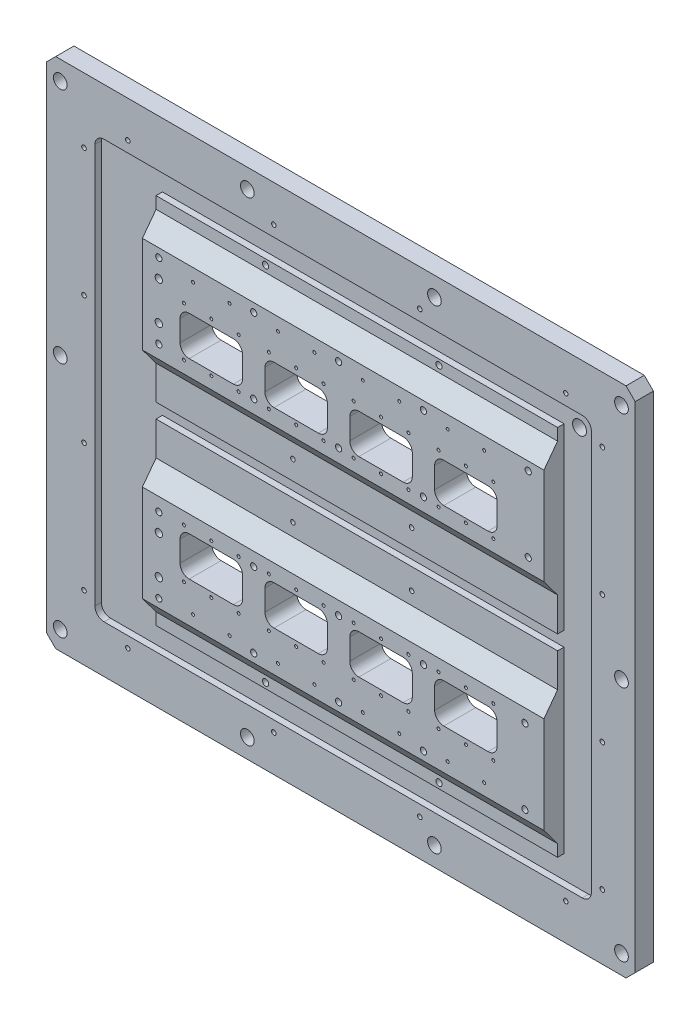
from build123d import *

# Parameters (mm, degrees)
SKETCH1_W             = 645
SKETCH1_H             = 562
BOSS_EXTRUDE1_DEPTH   = 20
SKETCH2_W             = 544
SKETCH2_H             = 458
CUT_EXTRUDE1_DEPTH    = 7
CHAMFER1_SIZE         = 10
BOSS_EXTRUDE2_DEPTH   = 440
CUT_EXTRUDE2_DEPTH    = 440
HOLE1_D               = 8.4
HOLE1_CBORE_D         = 15
HOLE1_CBORE_DEPTH     = 11
FILLET1_R             = 10
M6_TAPPED_HOLE1_D     = 5
M6_TAPPED_HOLE1_DEPTH = 10
M6_TAPPED_HOLE1_TIP   = 1.502151548
G3_8_TAPPED_HOLE1_D   = 15.25
M8_TAPPED_HOLE1_D     = 6.8
M8_TAPPED_HOLE1_DEPTH = 16
M8_TAPPED_HOLE1_TIP   = 2.042926105
HOLE2_D               = 8
HOLE2_DEPTH           = 8.5
M8_TAPPED_HOLE2_D     = 6.8
M8_TAPPED_HOLE2_DEPTH = 16
M8_TAPPED_HOLE2_TIP   = 2.042926105
M4_TAPPED_HOLE1_D     = 3.3
M4_TAPPED_HOLE1_DEPTH = 8
M4_TAPPED_HOLE1_TIP   = 0.991420021
M4_TAPPED_HOLE2_D     = 3.3
M4_TAPPED_HOLE2_DEPTH = 8
M4_TAPPED_HOLE2_TIP   = 0.991420021
M6_TAPPED_HOLE2_D     = 5
M6_TAPPED_HOLE2_DEPTH = 12
M6_TAPPED_HOLE2_TIP   = 1.502151548
M8_TAPPED_HOLE3_D     = 6.8
M8_TAPPED_HOLE3_DEPTH = 16
M8_TAPPED_HOLE3_TIP   = 2.042926105


with BuildPart() as part:
    # Sketch1 → Boss-Extrude1 (new body)
    with BuildSketch(Plane.XY):
        Rectangle(SKETCH1_W, SKETCH1_H)
    extrude(amount=BOSS_EXTRUDE1_DEPTH)

    # Sketch2 → Cut-Extrude1 (cut)
    with BuildSketch(Plane.XY.offset(20)):
        with Locations((2.5, 0)):
            Rectangle(SKETCH2_W, SKETCH2_H)
    extrude(amount=-CUT_EXTRUDE1_DEPTH, mode=Mode.SUBTRACT)

    # Chamfer1
    chamfer1_edges = [part.edges().sort_by_distance(p)[0] for p in [
        (322.5, -281, 10),
        (-322.5, -281, 10),
        (-322.5, 281, 10),
        (322.5, 281, 10),
    ]]
    chamfer(chamfer1_edges, length=CHAMFER1_SIZE)

    # Sketch3 → Boss-Extrude2 (add)
    with BuildSketch(Plane(origin=(-202.5, 0, 0), x_dir=(0, 0, -1), z_dir=(1, 0, 0))):
        Polygon((-13, 204), (-20, 204), (-20, 191), (-35, 171), (-35, 65), (-20, 45), (-20, 8), (-13, 8), align=None)
        Polygon((-20, -8), (-20, -45), (-35, -65), (-35, -171), (-20, -191), (-20, -204), (-13, -204), (-13, -8), align=None)
    extrude(amount=BOSS_EXTRUDE2_DEPTH)

    # Sketch4 → Cut-Extrude2 (cut)
    with BuildSketch(Plane.XY.offset(35)):
        with BuildLine():
            Line((-151.25, -83.74), (-102.75, -83.74))
            ThreePointArc((-102.75, -83.74), (-95.678932188, -86.668932188), (-92.75, -93.74))
            Line((-92.75, -93.74), (-92.75, -116.74))
            ThreePointArc((-92.75, -116.74), (-95.678932188, -123.811067812), (-102.75, -126.74))
            Line((-102.75, -126.74), (-151.25, -126.74))
            ThreePointArc((-151.25, -126.74), (-158.321067812, -123.811067812), (-161.25, -116.74))
            Line((-161.25, -116.74), (-161.25, -93.74))
            ThreePointArc((-161.25, -93.74), (-158.321067812, -86.668932188), (-151.25, -83.74))
        make_face()
        with BuildLine():
            Line((-68.25, -93.74), (-68.25, -116.74))
            ThreePointArc((-68.25, -116.74), (-65.321067812, -123.811067812), (-58.25, -126.74))
            Line((-58.25, -126.74), (-9.75, -126.74))
            ThreePointArc((-9.75, -126.74), (-2.678932188, -123.811067812), (0.25, -116.74))
            Line((0.25, -116.74), (0.25, -93.74))
            ThreePointArc((0.25, -93.74), (-2.678932188, -86.668932188), (-9.75, -83.74))
            Line((-9.75, -83.74), (-58.25, -83.74))
            ThreePointArc((-58.25, -83.74), (-65.321067812, -86.668932188), (-68.25, -93.74))
        make_face()
        with BuildLine():
            Line((24.75, -93.74), (24.75, -116.74))
            ThreePointArc((24.75, -116.74), (27.678932188, -123.811067812), (34.75, -126.74))
            Line((34.75, -126.74), (83.25, -126.74))
            ThreePointArc((83.25, -126.74), (90.321067812, -123.811067812), (93.25, -116.74))
            Line((93.25, -116.74), (93.25, -93.74))
            ThreePointArc((93.25, -93.74), (90.321067812, -86.668932188), (83.25, -83.74))
            Line((83.25, -83.74), (34.75, -83.74))
            ThreePointArc((34.75, -83.74), (27.678932188, -86.668932188), (24.75, -93.74))
        make_face()
        with BuildLine():
            Line((117.75, -93.74), (117.75, -116.74))
            ThreePointArc((117.75, -116.74), (120.678932188, -123.811067812), (127.75, -126.74))
            Line((127.75, -126.74), (176.25, -126.74))
            ThreePointArc((176.25, -126.74), (183.321067812, -123.811067812), (186.25, -116.74))
            Line((186.25, -116.74), (186.25, -93.74))
            ThreePointArc((186.25, -93.74), (183.321067812, -86.668932188), (176.25, -83.74))
            Line((176.25, -83.74), (127.75, -83.74))
            ThreePointArc((127.75, -83.74), (120.678932188, -86.668932188), (117.75, -93.74))
        make_face()
        with BuildLine():
            Line((-68.25, 115.5), (-68.25, 92.5))
            ThreePointArc((-68.25, 92.5), (-65.321067812, 85.428932188), (-58.25, 82.5))
            Line((-58.25, 82.5), (-9.75, 82.5))
            ThreePointArc((-9.75, 82.5), (-2.678932188, 85.428932188), (0.25, 92.5))
            Line((0.25, 92.5), (0.25, 115.5))
            ThreePointArc((0.25, 115.5), (-2.678932188, 122.571067812), (-9.75, 125.5))
            Line((-9.75, 125.5), (-58.25, 125.5))
            ThreePointArc((-58.25, 125.5), (-65.321067812, 122.571067812), (-68.25, 115.5))
        make_face()
        with BuildLine():
            Line((24.75, 115.5), (24.75, 92.5))
            ThreePointArc((24.75, 92.5), (27.678932188, 85.428932188), (34.75, 82.5))
            Line((34.75, 82.5), (83.25, 82.5))
            ThreePointArc((83.25, 82.5), (90.321067812, 85.428932188), (93.25, 92.5))
            Line((93.25, 92.5), (93.25, 115.5))
            ThreePointArc((93.25, 115.5), (90.321067812, 122.571067812), (83.25, 125.5))
            Line((83.25, 125.5), (34.75, 125.5))
            ThreePointArc((34.75, 125.5), (27.678932188, 122.571067812), (24.75, 115.5))
        make_face()
        with BuildLine():
            Line((117.75, 115.5), (117.75, 92.5))
            ThreePointArc((117.75, 92.5), (120.678932188, 85.428932188), (127.75, 82.5))
            Line((127.75, 82.5), (176.25, 82.5))
            ThreePointArc((176.25, 82.5), (183.321067812, 85.428932188), (186.25, 92.5))
            Line((186.25, 92.5), (186.25, 115.5))
            ThreePointArc((186.25, 115.5), (183.321067812, 122.571067812), (176.25, 125.5))
            Line((176.25, 125.5), (127.75, 125.5))
            ThreePointArc((127.75, 125.5), (120.678932188, 122.571067812), (117.75, 115.5))
        make_face()
        with BuildLine():
            Line((-161.25, 115.5), (-161.25, 92.5))
            ThreePointArc((-161.25, 92.5), (-158.321067812, 85.428932188), (-151.25, 82.5))
            Line((-151.25, 82.5), (-102.75, 82.5))
            ThreePointArc((-102.75, 82.5), (-95.678932188, 85.428932188), (-92.75, 92.5))
            Line((-92.75, 92.5), (-92.75, 115.5))
            ThreePointArc((-92.75, 115.5), (-95.678932188, 122.571067812), (-102.75, 125.5))
            Line((-102.75, 125.5), (-151.25, 125.5))
            ThreePointArc((-151.25, 125.5), (-158.321067812, 122.571067812), (-161.25, 115.5))
        make_face()
    extrude(amount=-CUT_EXTRUDE2_DEPTH, mode=Mode.SUBTRACT)

    # Hole1 (through all)
    with Locations(Plane.XY.offset(20)):
        with Locations((-307.5, 260), (-102.5, 260), (102.5, 260), (307.5, 260), (307.5, 0), (307.5, -260), (102.5, -260), (-102.5, -260), (-307.5, -260), (-307.5, 0)):
            CounterBoreHole(HOLE1_D / 2, HOLE1_CBORE_D / 2, HOLE1_CBORE_DEPTH)

    # Fillet1
    fillet1_edges = [part.edges().sort_by_distance(p)[0] for p in [
        (-269.5, -229, 16.5),
        (-269.5, 229, 16.5),
        (274.5, 229, 16.5),
        (274.5, -229, 16.5),
    ]]
    fillet(fillet1_edges, radius=FILLET1_R)

    # M6 Tapped Hole1
    with Locations(Plane.XY.offset(20)):
        with Locations((-281.5, -210), (-233.5, -241), (-73.5, -241), (86.5, -241), (246.5, -241), (286.5, 70), (286.5, 210), (246.5, 241), (86.5, 241), (-73.5, 241), (-233.5, 241), (-281.5, 210), (-281.5, 70), (286.5, -210), (286.5, -70), (-281.5, -70)):
            Hole(M6_TAPPED_HOLE1_D / 2, depth=M6_TAPPED_HOLE1_DEPTH)
            with Locations((0, 0, -(M6_TAPPED_HOLE1_DEPTH + M6_TAPPED_HOLE1_TIP / 2))):  # 118° drill point
                Cone(0, M6_TAPPED_HOLE1_D / 2, M6_TAPPED_HOLE1_TIP, mode=Mode.SUBTRACT)

    # G3/8 Tapped Hole1 (through all)
    with Locations(Plane.XY.offset(13)):
        with Locations((254.5, 209)):
            Hole(G3_8_TAPPED_HOLE1_D / 2)

    # M8 Tapped Hole1
    with Locations(Plane(origin=(0, 0, 0), x_dir=(-1, 0, 0), z_dir=(0, 0, -1))):
        with Locations((-212.5, 170), (-112.5, 170), (-12.5, 170), (87.5, 170), (187.5, 170), (187.5, 28), (87.5, 28), (-12.5, 28), (-112.5, 28), (-212.5, 28), (-212.5, -24), (-212.5, -166), (-112.5, -166), (-112.5, -24), (-12.5, -24), (87.5, -24), (187.5, -24), (187.5, -166), (87.5, -166), (-12.5, -166)):
            Hole(M8_TAPPED_HOLE1_D / 2, depth=M8_TAPPED_HOLE1_DEPTH)
            with Locations((0, 0, -(M8_TAPPED_HOLE1_DEPTH + M8_TAPPED_HOLE1_TIP / 2))):  # 118° drill point
                Cone(0, M8_TAPPED_HOLE1_D / 2, M8_TAPPED_HOLE1_TIP, mode=Mode.SUBTRACT)

    # Hole2
    with Locations(Plane.XY.offset(35)):
        with Locations((-184.5, 141.6), (-184.5, 99.6), (-184.5, -99.6), (-184.5, -141.6)):
            Hole(HOLE2_D / 2, depth=HOLE2_DEPTH)

    # M8 Tapped Hole2
    with Locations(Plane.XY.offset(35)):
        with Locations((-184.5, 161.6), (-80.5, 161.6), (12.5, 161.6), (105.5, 161.6), (220.3, 161.6), (220.3, 79.6), (105.5, 79.6), (12.5, 79.6), (-80.5, 79.6), (-184.5, 79.6), (-184.5, -79.6), (-184.5, -161.6), (-80.5, -161.6), (-80.5, -79.6), (12.5, -79.6), (12.5, -161.6), (105.5, -161.6), (105.5, -79.6), (216.7, -79.6), (216.7, -161.6)):
            Hole(M8_TAPPED_HOLE2_D / 2, depth=M8_TAPPED_HOLE2_DEPTH)
            with Locations((0, 0, -(M8_TAPPED_HOLE2_DEPTH + M8_TAPPED_HOLE2_TIP / 2))):  # 118° drill point
                Cone(0, M8_TAPPED_HOLE2_D / 2, M8_TAPPED_HOLE2_TIP, mode=Mode.SUBTRACT)

    # M4 Tapped Hole1
    with Locations(Plane.XY.offset(35)):
        with Locations((-147, 157), (-107, 157), (-54, 157), (-14, 157), (39, 157), (79, 157), (132, 157), (172, 157), (-147, -158.24), (-107, -158.24), (-54, -158.24), (-14, -158.24), (39, -158.24), (79, -158.24), (132, -158.24), (172, -158.24)):
            Hole(M4_TAPPED_HOLE1_D / 2, depth=M4_TAPPED_HOLE1_DEPTH)
            with Locations((0, 0, -(M4_TAPPED_HOLE1_DEPTH + M4_TAPPED_HOLE1_TIP / 2))):  # 118° drill point
                Cone(0, M4_TAPPED_HOLE1_D / 2, M4_TAPPED_HOLE1_TIP, mode=Mode.SUBTRACT)

    # M4 Tapped Hole2
    with Locations(Plane.XY.offset(35)):
        with Locations((-157, -78.24), (-127, -78.24), (-97, -78.24), (-157, -132.24), (-127, -132.24), (-97, -132.24), (-64, -78.24), (-34, -78.24), (-4, -78.24), (-34, -132.24), (-64, -132.24), (-4, -132.24), (29, -78.24), (59, -78.24), (89, -78.24), (122, -78.24), (122, -132.24), (89, -132.24), (59, -132.24), (29, -132.24), (152, -78.24), (182, -78.24), (182, -132.24), (152, -132.24), (-157, 132.24), (-157, 78.24), (-127, 78.24), (-97, 78.24), (-97, 132.24), (-127, 132.24), (-64, 132.24), (-34, 132.24), (-4, 132.24), (29, 132.24), (59, 132.24), (89, 132.24), (89, 78.24), (59, 78.24), (29, 78.24), (-4, 78.24), (-34, 78.24), (-64, 78.24), (122, 132.24), (122, 78.24), (152, 78.24), (182, 78.24), (152, 132.24), (182, 132.24)):
            Hole(M4_TAPPED_HOLE2_D / 2, depth=M4_TAPPED_HOLE2_DEPTH)
            with Locations((0, 0, -(M4_TAPPED_HOLE2_DEPTH + M4_TAPPED_HOLE2_TIP / 2))):  # 118° drill point
                Cone(0, M4_TAPPED_HOLE2_D / 2, M4_TAPPED_HOLE2_TIP, mode=Mode.SUBTRACT)

    # M6 Tapped Hole2
    with Locations(Plane.XY.offset(20)):
        with Locations((-52.5, 29), (-52.5, -31), (77.5, -31), (77.5, 29)):
            Hole(M6_TAPPED_HOLE2_D / 2, depth=M6_TAPPED_HOLE2_DEPTH)
            with Locations((0, 0, -(M6_TAPPED_HOLE2_DEPTH + M6_TAPPED_HOLE2_TIP / 2))):  # 118° drill point
                Cone(0, M6_TAPPED_HOLE2_D / 2, M6_TAPPED_HOLE2_TIP, mode=Mode.SUBTRACT)

    # M8 Tapped Hole3
    with Locations(Plane.XY.offset(20)):
        with Locations((-82.5, -198), (107.5, -198), (-82.5, 198), (107.5, 198)):
            Hole(M8_TAPPED_HOLE3_D / 2, depth=M8_TAPPED_HOLE3_DEPTH)
            with Locations((0, 0, -(M8_TAPPED_HOLE3_DEPTH + M8_TAPPED_HOLE3_TIP / 2))):  # 118° drill point
                Cone(0, M8_TAPPED_HOLE3_D / 2, M8_TAPPED_HOLE3_TIP, mode=Mode.SUBTRACT)


solid = part.part
